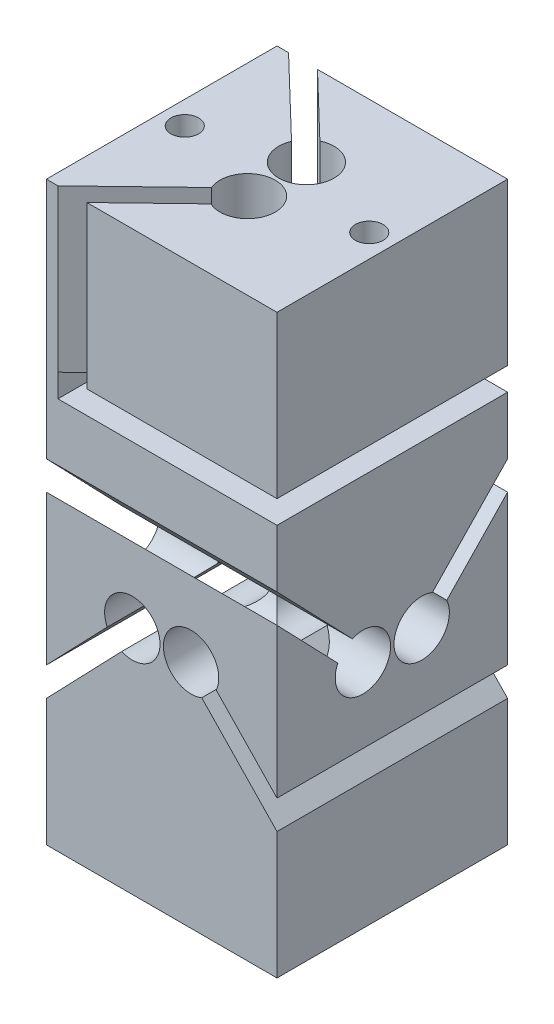
from build123d import *

# Parameters (mm, degrees)
SKETCH1_W           = 10
SKETCH1_H           = 10
BOSS_EXTRUDE1_DEPTH = 10
CUT_EXTRUDE1_DEPTH  = 16
CUT_EXTRUDE2_DEPTH  = 16
SKETCH4_W           = 10
SKETCH4_H           = 10
BOSS_EXTRUDE2_DEPTH = 5
SKETCH5_W           = 10
SKETCH5_H           = 10
BOSS_EXTRUDE3_DEPTH = 10
CUT_EXTRUDE3_DEPTH  = 8
SKETCH8_W           = 10
SKETCH8_H           = 1
CUT_EXTRUDE4_DEPTH  = 9.5
SKETCH10_R          = 1
CUT_EXTRUDE5_DEPTH  = 5
SKETCH11_R          = 0.6
CUT_EXTRUDE6_DEPTH  = 5


with BuildPart() as part:
    # Sketch1 → Boss-Extrude1 (new body)
    with BuildSketch(Plane(origin=(0, 0, 0), x_dir=(1, 0, 0), z_dir=(0, 1, 0))):
        Rectangle(SKETCH1_W, SKETCH1_H)
    extrude(amount=BOSS_EXTRUDE1_DEPTH)

    # Sketch2 → Cut-Extrude1 (cut, through all)
    with BuildSketch(Plane.XY.offset(5)):
        with BuildLine():
            Line((2.363818154, 4.495544821), (5, 1.754964793))
            Line((5, 1.754964793), (5, 0.5))
            Line((5, 0.5), (1.736808704, 3.892420332))
            ThreePointArc((1.736808704, 3.892420332), (0.443104153, 5.864840621), (2.363818154, 4.495544821))
        make_face()
        with BuildLine():
            Line((-5, 1.754964793), (-5, 0.5))
            Line((-5, 0.5), (-1.736808704, 3.892420332))
            ThreePointArc((-1.736808704, 3.892420332), (-0.443104153, 5.864840621), (-2.363818154, 4.495544821))
            Line((-2.363818154, 4.495544821), (-5, 1.754964793))
        make_face()
    extrude(amount=-CUT_EXTRUDE1_DEPTH, mode=Mode.SUBTRACT)

    # Sketch3 → Cut-Extrude2 (cut, through all)
    with BuildSketch(Plane(origin=(5, 0, 0), x_dir=(0, 0, -1), z_dir=(1, 0, 0))):
        with BuildLine():
            Line((2.363818154, 5.504455179), (5, 8.245035207))
            Line((5, 8.245035207), (5, 9.5))
            Line((5, 9.5), (1.736808704, 6.107579668))
            ThreePointArc((1.736808704, 6.107579668), (0.443104153, 4.135159379), (2.363818154, 5.504455179))
        make_face()
        with BuildLine():
            Line((-5, 9.5), (-5, 8.245035207))
            Line((-5, 8.245035207), (-2.363818154, 5.504455179))
            ThreePointArc((-2.363818154, 5.504455179), (-0.443104153, 4.135159379), (-1.736808704, 6.107579668))
            Line((-1.736808704, 6.107579668), (-5, 9.5))
        make_face()
    extrude(amount=-CUT_EXTRUDE2_DEPTH, mode=Mode.SUBTRACT)

    # Sketch4 → Boss-Extrude2 (add)
    with BuildSketch(Plane.XZ):
        Rectangle(SKETCH4_W, SKETCH4_H)
    extrude(amount=BOSS_EXTRUDE2_DEPTH)

    # Sketch5 → Boss-Extrude3 (add)
    with BuildSketch(Plane(origin=(0, 10, 0), x_dir=(1, 0, 0), z_dir=(0, 1, 0))):
        Rectangle(SKETCH5_W, SKETCH5_H)
    extrude(amount=BOSS_EXTRUDE3_DEPTH)

    # Sketch7 → Cut-Extrude3 (cut)
    with BuildSketch(Plane(origin=(0, 20, 0), x_dir=(1, 0, 0), z_dir=(0, 1, 0))):
        with BuildLine():
            Line((-0.504455179, -2.363818154), (-3.245035207, -5))
            Line((-3.245035207, -5), (-4.5, -5))
            Line((-4.5, -5), (-1.107579668, -1.736808704))
            ThreePointArc((-1.107579668, -1.736808704), (0.864840621, -0.443104153), (-0.504455179, -2.363818154))
        make_face()
        with BuildLine():
            Line((-3.245035207, 5), (-4.5, 5))
            Line((-4.5, 5), (-1.107579668, 1.736808704))
            ThreePointArc((-1.107579668, 1.736808704), (0.864840621, 0.443104153), (-0.504455179, 2.363818154))
            Line((-0.504455179, 2.363818154), (-3.245035207, 5))
        make_face()
    extrude(amount=-CUT_EXTRUDE3_DEPTH, mode=Mode.SUBTRACT)

    # Sketch8 → Cut-Extrude4 (cut)
    with BuildSketch(Plane(origin=(5, 0, 0), x_dir=(0, 0, -1), z_dir=(1, 0, 0))):
        with Locations((0, 12.5)):
            Rectangle(SKETCH8_W, SKETCH8_H)
    extrude(amount=-CUT_EXTRUDE4_DEPTH, mode=Mode.SUBTRACT)

    # Sketch10 → Cut-Extrude5 (cut)
    with BuildSketch(Plane.XZ.offset(5)):
        with Locations(Location((-2.828427125, 2.828427125, 0), (0, 0, 270))):
            Circle(SKETCH10_R)
        with Locations(Location((2.828427125, 2.828427125, 0), (0, 0, 270))):
            Circle(SKETCH10_R)
        with Locations(Location((2.828427125, -2.828427125, 0), (0, 0, 270))):
            Circle(SKETCH10_R)
        with Locations(Location((-2.828427125, -2.828427125, 0), (0, 0, 270))):
            Circle(SKETCH10_R)
    extrude(amount=-CUT_EXTRUDE5_DEPTH, mode=Mode.SUBTRACT)

    # Sketch11 → Cut-Extrude6 (cut)
    with BuildSketch(Plane(origin=(0, 20, 0), x_dir=(1, 0, 0), z_dir=(0, 1, 0))):
        with Locations(Location((4, 0, 0), (0, 0, 270))):
            Circle(SKETCH11_R)
        with Locations(Location((-4, 0, 0), (0, 0, 270))):
            Circle(SKETCH11_R)
    extrude(amount=-CUT_EXTRUDE6_DEPTH, mode=Mode.SUBTRACT)


solid = part.part
